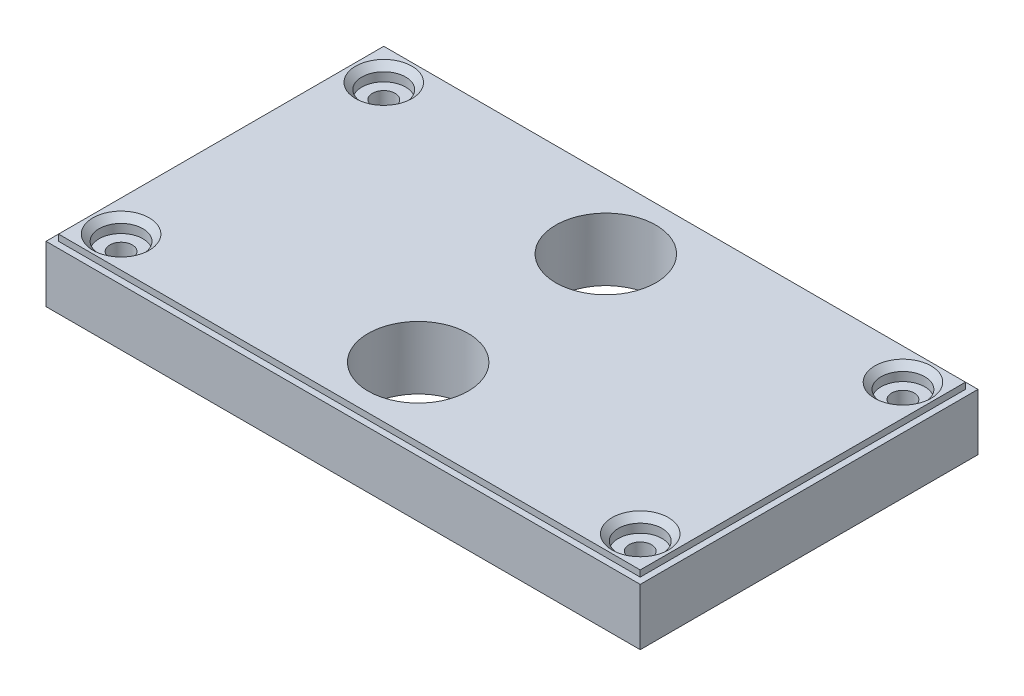
from build123d import *

# Parameters (mm, degrees)
SKETCH1_W                                = 95
SKETCH1_H                                = 54
BOSS_EXTRUDE1_DEPTH                      = 10.05
SKETCH2_OUTSIDE_W                        = 118.948
SKETCH2_OUTSIDE_H                        = 77.948
SKETCH2_OUTSIDE_W_2                      = 93
SKETCH2_OUTSIDE_H_2                      = 52
CUT_EXTRUDE1_DEPTH                       = 1
CBORE_FOR_M3_PAN_HEAD_SCREW1_D           = 3.6
CBORE_FOR_M3_PAN_HEAD_SCREW1_CBORE_D     = 7
CBORE_FOR_M3_PAN_HEAD_SCREW1_CBORE_DEPTH = 2.4
CHAMFER1_SIZE                            = 1
CUT_EXTRUDE2_REACH                       = 111.736
SKETCH5_R                                = 8


with BuildPart() as part:
    # Sketch1 → Boss-Extrude1 (new body)
    with BuildSketch(Plane(origin=(0, 0, 0), x_dir=(1, 0, 0), z_dir=(0, 1, 0))):
        with Locations((47.5, 27)):
            Rectangle(SKETCH1_W, SKETCH1_H)
    extrude(amount=BOSS_EXTRUDE1_DEPTH)

    # Sketch2 outside → Cut-Extrude1 (cut)
    with BuildSketch(Plane(origin=(0, 10.05, 0), x_dir=(1, 0, 0), z_dir=(0, 1, 0))):
        with Locations((47.5, 27)):
            Rectangle(SKETCH2_OUTSIDE_W, SKETCH2_OUTSIDE_H)
        with Locations((47.5, 27)):
            Rectangle(SKETCH2_OUTSIDE_W_2, SKETCH2_OUTSIDE_H_2, mode=Mode.SUBTRACT)
    extrude(amount=-CUT_EXTRUDE1_DEPTH, mode=Mode.SUBTRACT)

    # CBORE for M3 Pan Head Screw1 (through all)
    with Locations(Plane(origin=(6, 10.05, -48), x_dir=(0, 0, 1), z_dir=(0, 1, 0))):
        with Locations((0, 0), (0, 83), (42, 83), (42, 0)):
            CounterBoreHole(CBORE_FOR_M3_PAN_HEAD_SCREW1_D / 2, CBORE_FOR_M3_PAN_HEAD_SCREW1_CBORE_D / 2, CBORE_FOR_M3_PAN_HEAD_SCREW1_CBORE_DEPTH)

    # Chamfer1
    chamfer1_edges = [part.edges().sort_by_distance(p)[0] for p in [
        (6, 10.05, -9.5),
        (89, 10.05, -9.5),
        (89, 10.05, -51.5),
        (6, 10.05, -51.5),
    ]]
    chamfer(chamfer1_edges, length=CHAMFER1_SIZE)

    # Sketch5 → Cut-Extrude2 (cut, up to next)
    with BuildSketch(Plane(origin=(0, 10.05, 0), x_dir=(1, 0, 0), z_dir=(0, 1, 0)), mode=Mode.PRIVATE) as cut_extrude2_sk1:
        with Locations(Location((47.5, 42, 0), (0, 0, 270))):
            Circle(SKETCH5_R)
    cut_extrude2_tool1 = extrude(cut_extrude2_sk1.sketch, amount=-CUT_EXTRUDE2_REACH, mode=Mode.PRIVATE) & part.part
    # Sketch5 → Cut-Extrude2 (cut, up to next)
    with BuildSketch(Plane(origin=(0, 10.05, 0), x_dir=(1, 0, 0), z_dir=(0, 1, 0)), mode=Mode.PRIVATE) as cut_extrude2_sk2:
        with Locations(Location((47.5, 12, 0), (0, 0, 270))):
            Circle(SKETCH5_R)
    cut_extrude2_tool2 = extrude(cut_extrude2_sk2.sketch, amount=-CUT_EXTRUDE2_REACH, mode=Mode.PRIVATE) & part.part
    add(cut_extrude2_tool1.solids().sort_by_distance((47.5, 10.05, -42))[0], mode=Mode.SUBTRACT)
    add(cut_extrude2_tool2.solids().sort_by_distance((47.5, 10.05, -12))[0], mode=Mode.SUBTRACT)


solid = part.part
